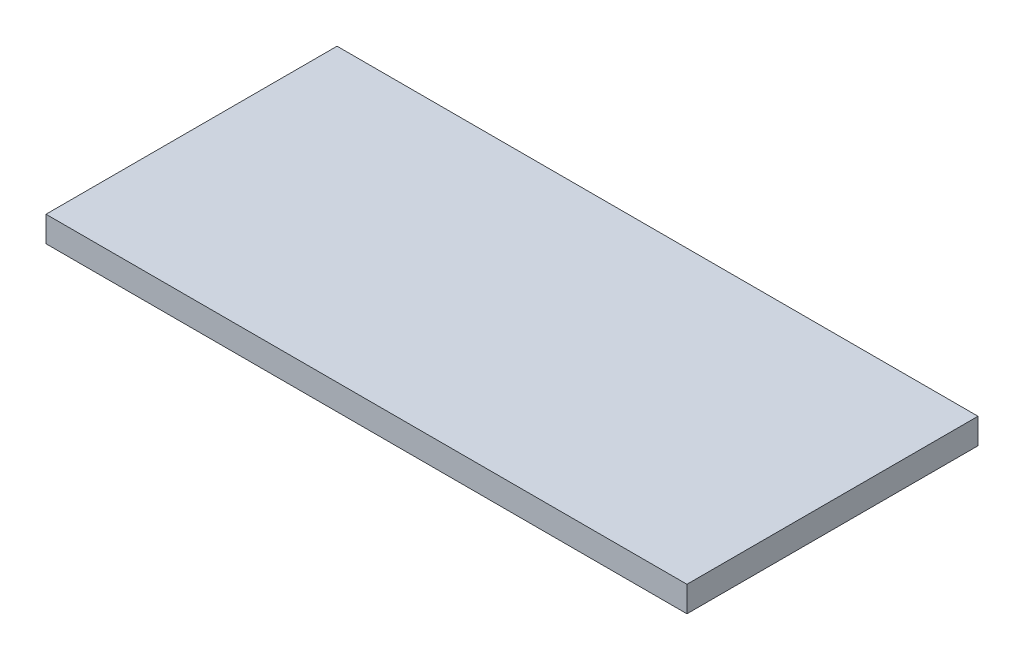
SolidWorks part; units mm, degrees
ref_plane "Front Plane" through (0, 0, 0) normal (0, 0, 1) x (1, 0, 0)
ref_plane "Top Plane" through (0, 0, 0) normal (0, 1, 0) x (1, 0, 0)
ref_plane "Right Plane" through (0, 0, 0) normal (1, 0, 0) x (0, 0, -1)
sketch "Sketch2" plane through (0, 0, 0) normal (1, 0, 0) x (0, 0, -1)
  line L1 (0, 0) -> (-455, 0)
  line L2 (-455, 0) -> (-455, -40)
  line L3 (0, 0) -> (0, -40)
  line L4 (0, -40) -> (-22, -40)
  line L5 (-22, -40) -> (-22, -50)
  dimension "D1" = 455
  dimension "D2" = 40
  dimension "D3" = 40
  dimension "D4" = 22
  dimension "D5" = 10
extrude "Extrude-Thin1" add sketch "Sketch2" along normal mid plane 1000 thin thin type one direction wall 1
sketch "Sketch3" plane through (500, 0, 0) normal (1, 0, 0) x (0, 0, -1)
  line L0 (-455, -40) -> (-455, 0)
  line L1 (-455, 0) -> (0, 0)
  line L2 (0, 0) -> (0, -40)
  line L3 (0, -40) -> (-455, -40)
extrude "Extrude1" add sketch "Sketch3" along normal blind 1
sketch "Sketch7" plane through (-500, 0, 0) normal (-1, 0, 0) x (0, 0, 1)
  line L0 (0, -40) -> (0, 0)
  line L1 (0, 0) -> (455, 0)
  line L2 (455, 0) -> (455, -40)
  line L3 (455, -40) -> (0, -40)
extrude "Extrude3" add sketch "Sketch7" along normal blind 1
sketch "Sketch8" plane through (0, -50, 0) normal (0, -1, 0) x (1, 0, 0)
  line L0 (500, 22) -> (-500, 22) construction
  line L1 (500, 23) -> (457, 23)
  line L2 (500, 23) -> (500, 22)
  line L3 (500, 22) -> (457, 22)
  line L4 (457, 23) -> (457, 22)
  line L5 (500, 23) -> (-500, 23) construction
  line L6 (-500, 22) -> (-457, 22)
  line L7 (-500, 22) -> (-500, 23)
  line L8 (-500, 23) -> (-457, 23)
  line L9 (-457, 22) -> (-457, 23)
  dimension "D1" = 43
  dimension "D2" = 43
extrude "Cut-Extrude1" cut sketch "Sketch8" against normal blind 20
sketch "Sketch9" plane through (0, -40, 0) normal (0, -1, 0) x (1, 0, 0)
  line L0 (501, 455) -> (501, 0) construction
  line L1 (501, 0) -> (-501, 0) construction
  line L2 (0, 0) -> (0, 693.9053) construction
  circle A0 centre (491, 15) radius 2.75
  circle A1 centre (-491, 15) radius 2.75
  dimension "D1" = 5.5
  dimension "D2" = 10
  dimension "D3" = 15
extrude "Cut-Extrude2" cut sketch "Sketch9" against normal blind 10
